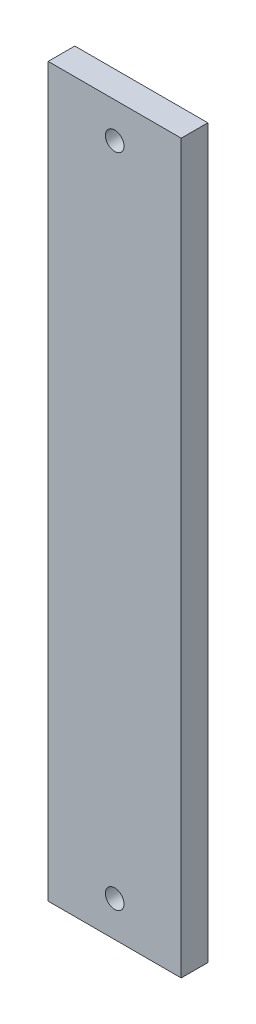
SolidWorks part; units mm, degrees
material "Q235"
ref_plane "Front Plane" through (0, 0, 0) normal (0, 0, 1) x (1, 0, 0)
ref_plane "Top Plane" through (0, 0, 0) normal (0, 1, 0) x (1, 0, 0)
ref_plane "Right Plane" through (0, 0, 0) normal (1, 0, 0) x (0, 0, -1)
sketch "Sketch1" plane through (0, 0, 0) normal (0, 0, 1) x (1, 0, 0)
  line L1 (0, 0) -> (150, 0)
  line L2 (0, 0) -> (0, 820)
  line L3 (0, 820) -> (150, 820)
  line L4 (150, 0) -> (150, 820)
  dimension "D1" = 820
  dimension "D2" = 150
extrude "Boss-Extrude1" add sketch "Sketch1" along normal blind 30
hole_wizard "M24 Threaded hole1" positions "3DSketch1" profile "Sketch2" tap size "M24" standard "GB" end condition through all
sketch3d "3DSketch1"
  line L0 (150, 0, 30) -> (150, 820, 30) construction
  line L1 (150, 820, 30) -> (0, 820, 30) construction
  point P0 (75, 780, 30)
  point P2 (75, 40, 30)
  point P11 (283.452, 183.2952, 0)
  dimension "D1" = 75
  dimension "D2" = 40
  dimension "D3" = 740
sketch "Sketch2" plane through (75, 780, 30) normal (1, 0, 0) x (0, -1, 0)
  line L0 (0, 0) -> (0, 30)
  line L1 (0, 30) -> (10.5, 30)
  line L2 (10.5, 30) -> (10.5, 0)
  line L5 (10.5, 0) -> (0, 0)
  line L11 (0, -6.35) -> (0, 107.95) construction
  dimension "通孔螺纹孔钻头直径" = 21
  dimension "通孔螺纹孔钻头深度" = 30
cosmetic thread "孔螺蚊线1" parameters "D2"=24
cosmetic thread "孔螺蚊线2" parameters "D2"=24
cosmetic thread "孔螺蚊线3" parameters "D2"=24
